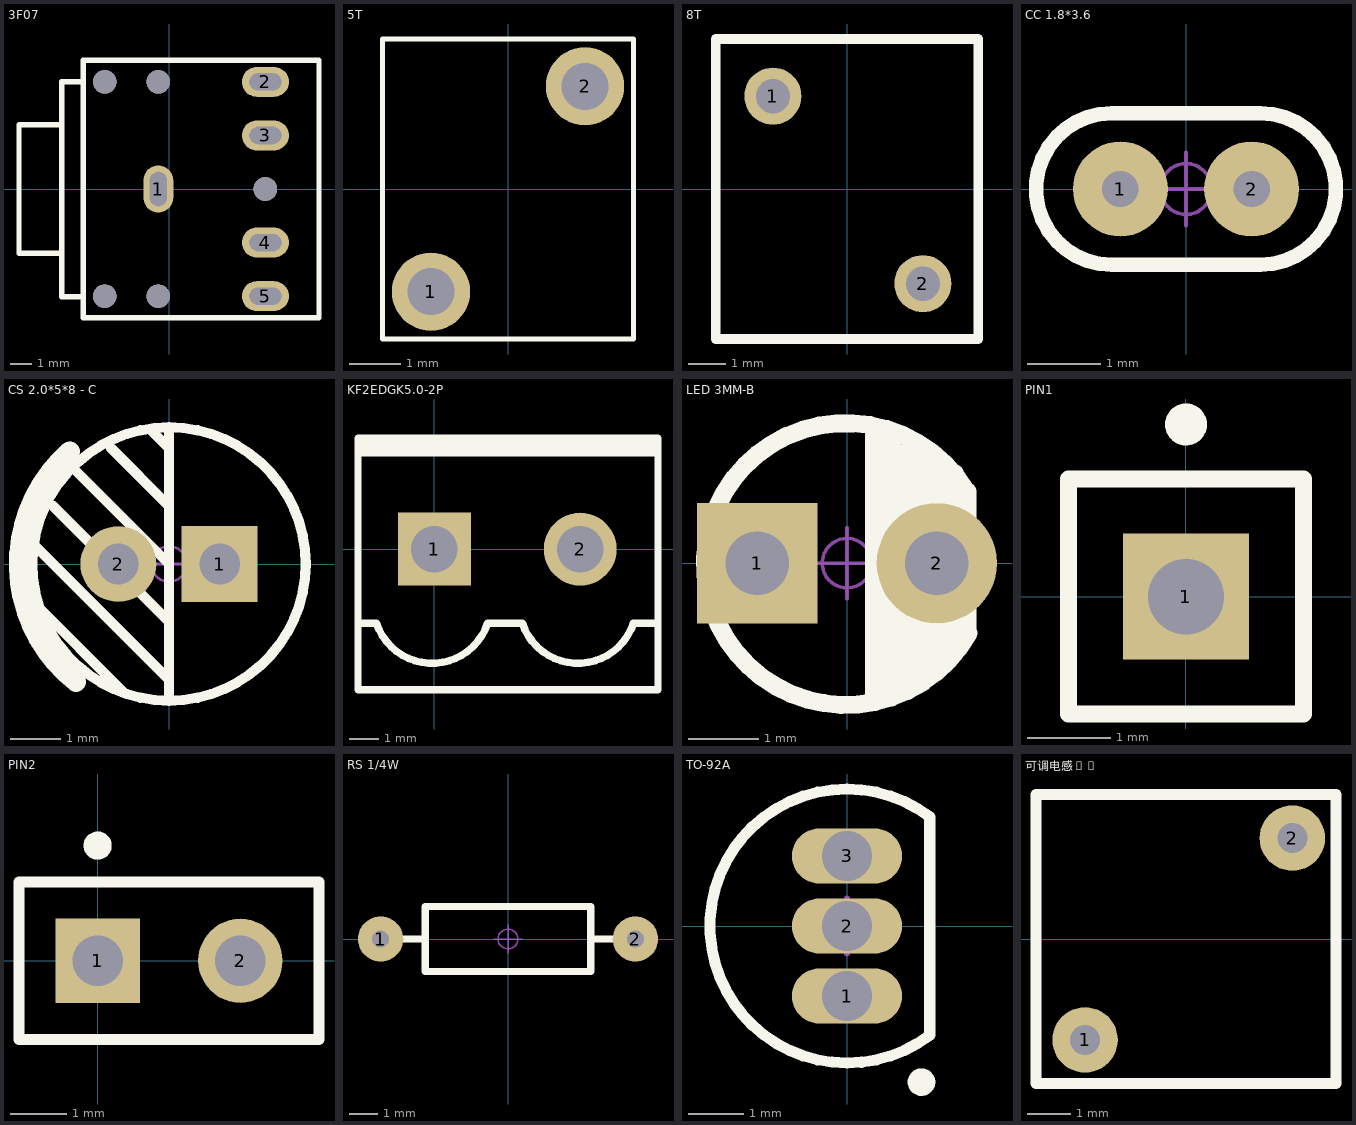
[diagram p0: the footprints below, top view; thin cyan lines are the x and y axes]
# Altium footprint library MISC80838.PcbLib: 12 footprints
Each footprint in its own frame and in the unit in brackets; x right, y up, seen from the top. Pads: shape width x height; smd on the part's side, far side on the other; paste and mask are expansions set on the pad; w line width, h text height; cw(c..) or ccw(c..) is an arc to the next point about the centre after c.

## 3F07 [mm]
pads (10):
  oval 1.4x2.2 hole 0.8 slot 1.6 at 90 deg paste+0 mask+0.051: 1(-0.5,0)
  oval 2.2x1.4 hole 0.8 slot 1.5 at 0 deg paste+0 mask+0.051: 2(4.5,5) 3(4.5,2.5) 4(4.5,-2.5) 5(4.5,-5)
  round 1.1 hole 1.1 unplated paste+0: ""(-3,-5) ""(-3,5) ""(-0.5,-5) ""(-0.5,5) ""(4.5,0)
Top Overlay:
  lines w0.254: -5,-3 -7,-3 -7,3 -5,3 ; -4,-5.026 -5,-5.026 -5,5 -4,5 ; -4,5 -4,-5 -4,-6 7,-6 7,6 -4,6 -4,5
Mechanical 15:
  circle w0.45: c-3,-5 r0.225
  circle w0.45: c-0.5,-5 r0.225
  circle w0.45: c-0.5,5 r0.225
  circle w0.45: c-3,5 r0.225
  circle w0.45: c4.5,0 r0.225

## 5T [mil]
pads (2):
  round 60 hole 36 paste+4 mask+4: 1(-59.05,-78.74) 2(59.05,78.74)
Top Overlay:
  lines w3.94: -96.25,-115 -96.25,115 96.25,115 96.25,-115 -96.25,-115

## 8T [mil]
pads (2):
  round 60 hole 36 paste+0 mask+2: 1(-77.8,97.48) 2(79.69,-99.37)
Top Overlay:
  lines w10: -137.79,-157.48 137.79,-157.48 137.79,157.48 -137.79,157.48 -137.79,-157.48

## CC 1.8*3.6 [mm]
pads (2):
  round 1.3 hole 0.5: 1(-0.9,0) 2(0.9,0)
Top Overlay:
  lines w0.2: -1.016,-1.041 cw(c-1.016,0) -1.016,1.041 1.016,1.041 cw(c1.016,0) 1.016,-1.041 -1.016,-1.041
Mechanical 15:
  circle w0.05: c0,0 r0.35
  lines w0.05: -0.5,0 0.5,0 ; 0,-0.5 0,0.5
3D body "CC 1.8X3.6.STEP": height 3.6, standoff -3.5, extent -1.8,-0.798 1.8,0.796

## CS 2.0*5*8 - C [mm]
pads (2):
  rect 1.5x1.5 hole 0.8: 1(1,0)
  round 1.5 hole 0.8: 2(-1,0)
Top Overlay:
  circle w0.2: c0,0 r2.7
  lines w0.2: -2.667,-0.762 -0.889,-2.54 ; -2.667,0.381 0,-2.286 ; -2.286,1.143 0,-1.143 ; -1.905,1.905 0,0 ; -1.143,2.286 0,1.143 ; -0.381,2.667 0,2.286 ; 0,-2.667 0,2.667
  lines w0.4: -1.96,2.221 ccw(c0,0) -1.835,-2.325
Mechanical 15:
  circle w0.05: c0,0 r0.35
  lines w0.05: -0.5,0 0.5,0 ; 0,-0.5 0,0.5
3D body "CS 5X8.STEP": height 8.02, standoff -3.48, extent -2.5,-2.5 2.5,2.5

## KF2EDGK5.0-2P [mm]
pads (2):
  rect 2.5x2.5 hole 1.6: 1(0,0)
  round 2.5 hole 1.6: 2(5,0)
Top Overlay:
  lines w0.254: -2.62,-2.54 -1.985,-2.54 ccw(c-0.08,-1.905) 1.825,-2.54 3.015,-2.54 ccw(c4.92,-1.905) 6.825,-2.54 7.667,-2.54 ; -2.62,3.302 7.667,3.302 ; -2.62,3.556 7.667,3.556 ; -2.62,-4.826 -2.62,3.81 7.667,3.81 7.667,-4.826 -2.62,-4.826
3D body "KF2EDGK5.0-LI.STEP": height 11.25, standoff -2.95, extent 2.46,-4.758 7.54,3.742
3D body "KF2EDGK5.0-LI.STEP": height 11.25, standoff -2.95, extent -2.54,-4.758 2.54,3.742

## LED 3MM-B [mm]
pads (2):
  rect 1.7x1.7 hole 0.9: 1(-1.27,0)
  round 1.7 hole 0.9: 2(1.27,0)
Top Overlay:
  lines w0.254: 0.381,-1.905 0.381,1.905 ; 0.635,-1.778 0.635,1.778 ; 1.016,-1.651 1.016,1.524 ; 1.524,1.27 1.524,-1.27 1.27,-1.524 1.27,1.397 1.143,1.524 1.016,1.524 ; 1.685,1.025 ccw(c-0.016,-0.012) 1.72,-0.987 ; 1.702,-0.965 1.702,1.016 ; 0.889,1.651 0.889,-1.778 0.889,1.651 ; 0.889,1.651 1.016,1.524
Mechanical 15:
  circle w0.05: c0,0 r0.35
  lines w0.05: -0.5,0 0.5,0 ; 0,-0.5 0,0.5
3D body "LED 3mm-玻璃罩.STEP": height 5.55, standoff 0.05, extent -1.95,-1.95 1.638,1.95
3D body "LED 3mm-B.STEP": height 3, standoff -3.45, extent -1.623,-0.838 1.618,0.838

## PIN1 [mm]
pads (1):
  rect 1.5x1.5 hole 0.9: 1(0,0)
Top Overlay:
  circle w0.25: c0,2.05 r0.125
  lines w0.2: -1.4,-1.4 1.4,-1.4 1.4,1.4 -1.4,1.4 -1.4,-1.4

## PIN2 [mm]
pads (2):
  rect 1.5x1.5 hole 0.9: 1(0,0)
  round 1.5 hole 0.9: 2(2.54,0)
Top Overlay:
  circle w0.25: c0,2.05 r0.125
  lines w0.2: -1.4,-1.4 3.94,-1.4 3.94,1.4 -1.4,1.4 -1.4,-1.4

## RS 1/4W [mm]
pads (2):
  round 1.6 hole 0.6: 1(-4.5,0) 2(4.5,0)
Top Overlay:
  lines w0.254: -3.683,0 -3.048,0 ; 3.048,0 3.683,0 ; -2.921,-1.143 2.921,-1.143 2.921,1.143 -2.921,1.143 -2.921,-1.143
Mechanical 15:
  circle w0.05: c0,0 r0.35
  lines w0.05: -0.5,0 0.5,0 ; 0,-0.5 0,0.5
3D body "RS 1-4W.STEP": height 2.32, standoff -3.49, extent -4.725,-1.16 4.725,1.16

## TO-92A [mm]
pads (3):
  oval 2x1 hole 0.9: 1(0,-1.27) 2(0,0) 3(0,1.27)
Top Overlay:
  circle w0.25: c1.35,-2.83 r0.125
  lines w0.2: 1.5,-1.98 cw(c0,0) 1.5,1.98 1.5,-1.98
Mechanical 13:
  lines w0.1: 1.5,-1.98 cw(c0,0) 1.5,1.98 1.5,-1.98
Mechanical 15:
  lines w0.1: -0.5,0 0.5,0 ; 0,-0.5 0,0.5
3D body: height 6.86, standoff 2.2, extent -2.485,-2.495 1.501,2.495

## 可调电感7T [mil]
pads (2):
  round 60 hole 27.56 paste+0 mask+2: 1(154.69,-92.5) 2(344.69,92.5)
Top Overlay:
  lines w10: 109.69,-132.5 384.69,-132.5 384.69,132.5 109.69,132.5 109.69,-132.5